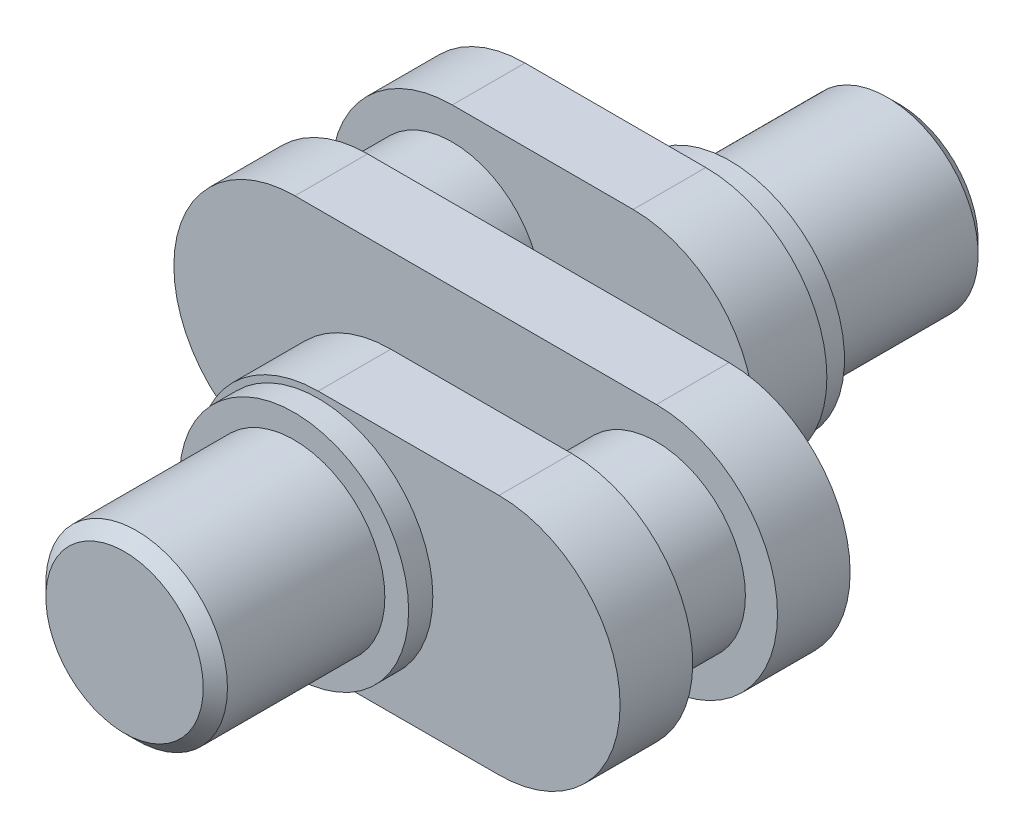
SolidWorks part; units mm, degrees
ref_plane "Front Plane" through (0, 0, 0) normal (0, 0, 1) x (1, 0, 0)
ref_plane "Top Plane" through (0, 0, 0) normal (0, 1, 0) x (1, 0, 0)
ref_plane "Right Plane" through (0, 0, 0) normal (1, 0, 0) x (0, 0, -1)
other "Configuration Table"
sketch "Sketch1" plane through (0, 0, 0) normal (0, 0, 1) x (1, 0, 0)
  line L0 (-7.4641, 5.0077) -> (7.4641, 5.0077)
  line L1 (-7.4641, -4.9923) -> (7.4641, -4.9923)
  arc A1 (7.4641, -4.9923) -> (7.4641, 5.0077) centre (7.4641, 0.0077) ccw
  arc A3 (-7.4641, 5.0077) -> (-7.4641, -4.9923) centre (-7.4641, 0.0077) ccw
extrude "Boss-Extrude7" add sketch "Sketch1" against normal up to surface (3 mm away)
sketch "Sketch7" plane through (0, 0, -3) normal (0, 0, -1) x (-1, 0, 0)
  circle A1 centre (7.4641, 0.0077) radius 3.6746
extrude "Boss-Extrude8" add sketch "Sketch7" along normal up to surface (3.5 mm away)
sketch "Sketch8" plane through (0, 0, 0) normal (0, 0, 1) x (1, 0, 0)
  circle A1 centre (7.4641, 0.0077) radius 3.6746
extrude "Boss-Extrude9" add sketch "Sketch8" along normal up to surface (3.5 mm away)
sketch "Sketch9" plane through (0, 0, -6.5) normal (0, 0, -1) x (-1, 0, 0)
  line L0 (-0.0039, 5.0039) -> (7.4641, 5.0077)
  line L1 (0.0039, -5) -> (7.4641, -4.9923)
  arc A0 (7.4641, -4.9923) -> (7.4589, 5.0077) centre (7.4641, 0.0077) ccw
  arc A1 (-0.0039, 5.0039) -> (0.0039, -5) centre (-0.0013, 0.0019) ccw
  circle M5 centre (7.4641, 0.0077) radius 3.6746
extrude "Boss-Extrude10" add sketch "Sketch9" along normal blind 3 contours L0 A1 L1 A0 M5 | M5
sketch "Sketch10" plane through (0, 0, 3.5) normal (0, 0, 1) x (1, 0, 0)
  line L0 (0.0043, -5) -> (7.3892, -4.9917)
  line L1 (-0.0039, 5.0039) -> (7.4641, 5.0077)
  arc A0 (7.3892, -4.9917) -> (7.4589, 5.0077) centre (7.4641, 0.0077) ccw
  arc A1 (-0.0039, 5.0039) -> (0.0043, -5) centre (-0.0013, 0.0019) ccw
  circle M3 centre (7.4641, 0.0077) radius 3.6746
extrude "Boss-Extrude11" add sketch "Sketch10" along normal blind 3 contours L1 A1 L0 A0 M3 | M3
sketch "Sketch11" plane through (0, 0, 6.5) normal (0, 0, 1) x (1, 0, 0)
  circle A0 centre (0, 0.0154) radius 4.7313
extrude "Boss-Extrude12" add sketch "Sketch11" along normal blind 1
sketch "Sketch12" plane through (0, 0, 7.5) normal (0, 0, 1) x (1, 0, 0)
  circle A0 centre (0, 0.0154) radius 3.75
extrude "Boss-Extrude13" add sketch "Sketch12" along normal blind 7
sketch "Sketch13" plane through (0, 0, -9.5) normal (0, 0, -1) x (-1, 0, 0)
  circle A1 centre (0, 0.0154) radius 4.7313
  circle A2 centre (0, 0.0154) radius 4.7313
  dimension "D1" = 0
extrude "Boss-Extrude14" add sketch "Sketch13" along normal blind 1
sketch "Sketch14" plane through (0, 0, -10.5) normal (0, 0, -1) x (-1, 0, 0)
  circle A1 centre (0, 0.0154) radius 3.75
  circle A2 centre (0, 0.0154) radius 3.75
  dimension "D1" = 0
extrude "Boss-Extrude15" add sketch "Sketch14" along normal blind 7
chamfer "Chamfer1" distance 0.5 angle 45 2 edges at (3.75, 0.0154, 14.5) (-3.75, 0.0154, -17.5)
